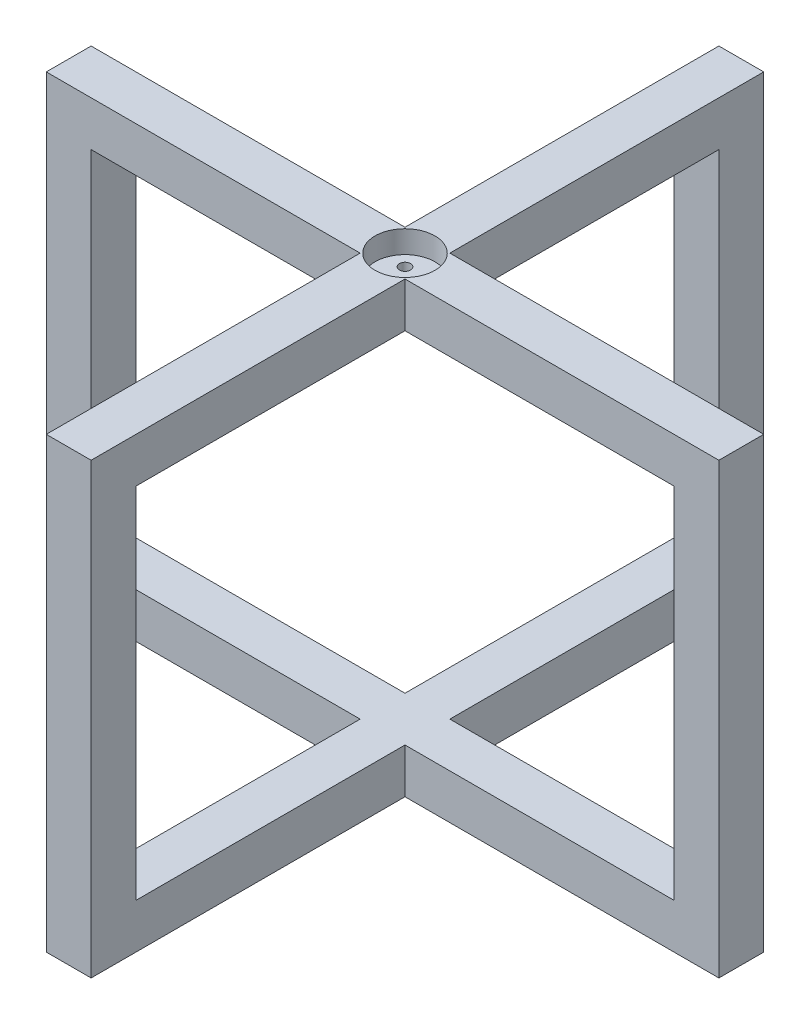
from build123d import *

# Parameters (mm, degrees)
SKETCH1_W                        = 900
SKETCH1_H                        = 600
SKETCH1_W_2                      = 780
SKETCH1_H_2                      = 480
BOSS_EXTRUDE1_DEPTH              = 30
SKETCH2_W                        = 900
SKETCH2_H                        = 600
SKETCH2_W_2                      = 780
SKETCH2_H_2                      = 480
BOSS_EXTRUDE2_DEPTH              = 30
SKETCH3_R                        = 40
CUT_EXTRUDE1_DEPTH               = 30
BLIND_DOWEL_HOLE_0_SIZE_MM_D     = 15
BLIND_DOWEL_HOLE_0_SIZE_MM_DEPTH = 100
BLIND_DOWEL_HOLE_0_SIZE_MM_TIP   = 4.506454643


with BuildPart() as part:
    # Sketch1 → Boss-Extrude1 (new, symmetric)
    with BuildSketch(Plane.XY):
        Rectangle(SKETCH1_W, SKETCH1_H)
        Rectangle(SKETCH1_W_2, SKETCH1_H_2, mode=Mode.SUBTRACT)
    extrude(amount=BOSS_EXTRUDE1_DEPTH, both=True)

    # Sketch2 → Boss-Extrude2 (add, symmetric)
    with BuildSketch(Plane(origin=(0, 0, 0), x_dir=(0, 0, -1), z_dir=(1, 0, 0))):
        Rectangle(SKETCH2_W, SKETCH2_H)
        Rectangle(SKETCH2_W_2, SKETCH2_H_2, mode=Mode.SUBTRACT)
    extrude(amount=BOSS_EXTRUDE2_DEPTH, both=True)

    # Sketch3 → Cut-Extrude1 (cut)
    with BuildSketch(Plane(origin=(0, 300, 0), x_dir=(1, 0, 0), z_dir=(0, 1, 0))):
        with Locations(Location((0, 0, 0), (0, 0, 270))):
            Circle(SKETCH3_R)
    extrude(amount=-CUT_EXTRUDE1_DEPTH, mode=Mode.SUBTRACT)

    # Blind dowel hole 0 (size mm)
    with Locations(Plane(origin=(0, 270, 0), x_dir=(1, 0, 0), z_dir=(0, 1, 0))):
        with Locations((-14.142135624, 14.142135624), (14.142135624, -14.142135624)):
            Hole(BLIND_DOWEL_HOLE_0_SIZE_MM_D / 2, depth=BLIND_DOWEL_HOLE_0_SIZE_MM_DEPTH)
            with Locations((0, 0, -(BLIND_DOWEL_HOLE_0_SIZE_MM_DEPTH + BLIND_DOWEL_HOLE_0_SIZE_MM_TIP / 2))):  # 118° drill point
                Cone(0, BLIND_DOWEL_HOLE_0_SIZE_MM_D / 2, BLIND_DOWEL_HOLE_0_SIZE_MM_TIP, mode=Mode.SUBTRACT)


solid = part.part
